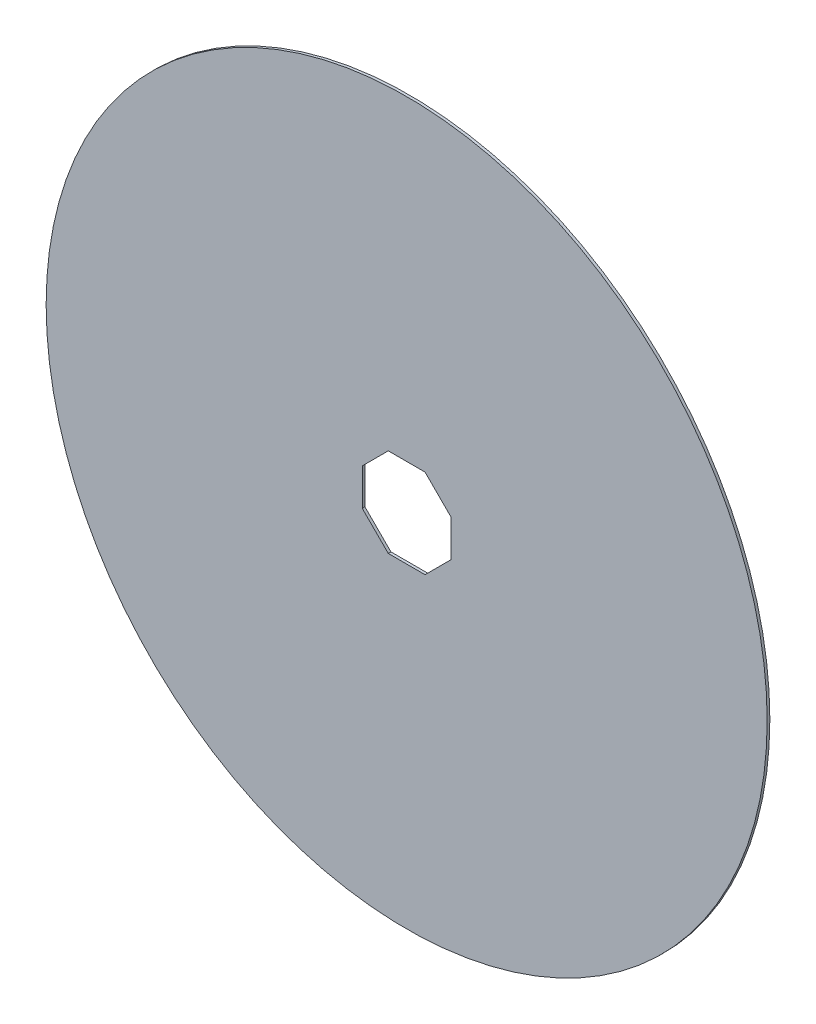
from build123d import *

# Parameters (mm, degrees)
SKETCH_1_R      = 270
EXTRUDE_1_DEPTH = 2


with BuildPart() as part:
    # 草图1 → 凸台-拉伸1 (new body)
    with BuildSketch(Plane.XY):
        Circle(SKETCH_1_R)
        Polygon((33.25966317, 13.776603565), (13.776603565, 33.25966317), (-13.776603565, 33.25966317), (-33.25966317, 13.776603565), (-33.25966317, -13.776603565), (-13.776603565, -33.25966317), (13.776603565, -33.25966317), (33.25966317, -13.776603565), align=None, mode=Mode.SUBTRACT)
    extrude(amount=EXTRUDE_1_DEPTH)


solid = part.part
